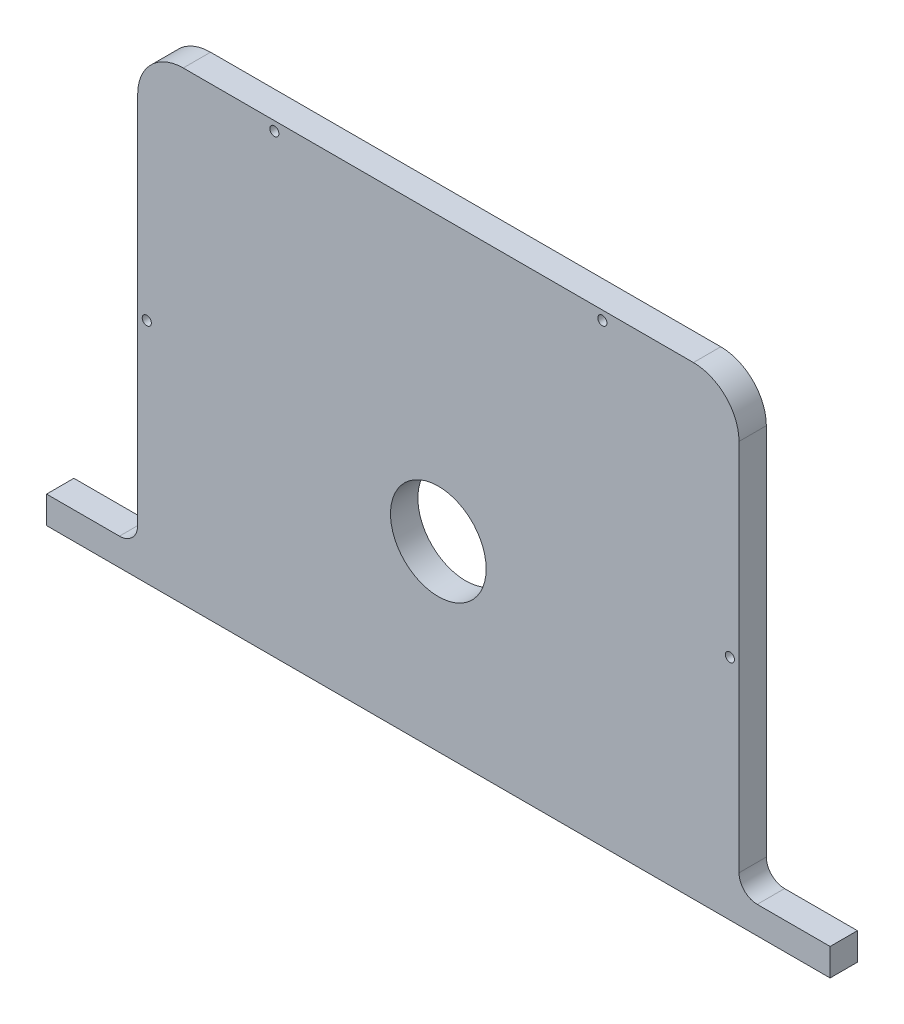
SolidWorks part; units mm, degrees
ref_plane "Front Plane" through (0, 0, 0) normal (0, 0, 1) x (1, 0, 0)
ref_plane "Top Plane" through (0, 0, 0) normal (0, 1, 0) x (1, 0, 0)
ref_plane "Right Plane" through (0, 0, 0) normal (1, 0, 0) x (0, 0, -1)
sketch "Sketch1" plane through (0, 0, 0) normal (0, 0, 1) x (1, 0, 0)
  line L1 (86, 0) -> (86, 3)
  line L2 (86, 3) -> (78, 3)
  line L3 (76, 5) -> (76, 46)
  line L4 (71, 51) -> (15, 51)
  line L5 (10, 46) -> (10, 5)
  line L6 (8, 3) -> (0, 3)
  line L7 (0, 3) -> (0, 0)
  line L8 (86, 0) -> (0, 0)
  arc A0 (78, 3) -> (76, 5) centre (78, 5) cw
  arc A1 (10, 5) -> (8, 3) centre (8, 5) cw
  arc A2 (76, 46) -> (71, 51) centre (71, 46) ccw
  arc A3 (15, 51) -> (10, 46) centre (15, 46) ccw
  circle A4 centre (43, 20) radius 5.25
  circle A5 centre (25, 50) radius 0.5
  circle A6 centre (61, 50) radius 0.5
  circle A7 centre (75, 25) radius 0.5
  circle A8 centre (11, 25) radius 0.5
  point P11 (76, 3)
  point P14 (10, 3)
  point P17 (76, 51)
  point P20 (10, 51)
  dimension "D7" = 2
  dimension "D8" = 5
  dimension "D9" = 10.5
  dimension "D10" = 20
  dimension "D11" = 33
  dimension "D12" = 1
  dimension "D13" = 1
  dimension "D14" = 1
  dimension "D15" = 1
  dimension "D16" = 1
  dimension "D17" = 1
  dimension "D18" = 1
  dimension "D19" = 1
  dimension "D20" = 15
  dimension "D21" = 15
  dimension "D22" = 26
  dimension "D23" = 26
  dimension "D1" = 66
  dimension "D2" = 10
  dimension "D3" = 10
  dimension "D4" = 48
  dimension "D5" = 48
  dimension "D6" = 3
extrude "Boss-Extrude1" add sketch "Sketch1" along normal blind 3
